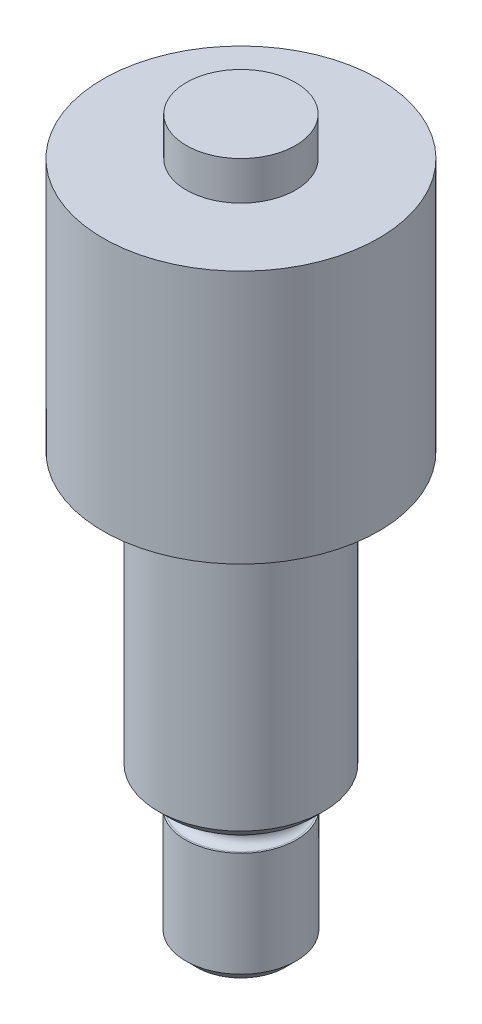
from build123d import *

# Parameters (mm, degrees)
CHAMFER_1_SIZE = 2
FILLET_1_R     = 1
FILLET_2_R     = 1.5


with BuildPart() as part:
    # 草图1 → 旋转1 (revolve)
    with BuildSketch(Plane.XY, mode=Mode.PRIVATE) as revolve_1_sk:
        Polygon((0, 0), (9.9, 0), (9.9, -7), (25, -7), (25, -53), (15, -53), (15, -104), (8.2, -104), (8.2, -109), (10, -109), (10, -130), (0, -130), align=None)
    revolve(revolve_1_sk.sketch.rotate(Axis((0, -130, 0), (0, 1, 0)), 90), axis=Axis((0, -130, 0), (0, 1, 0)))

    # 倒角1
    chamfer_1_edges = [part.edges().sort_by_distance(p)[0] for p in [
        (0, -104, 15),
        (0, -130, 10),
    ]]
    chamfer(chamfer_1_edges, length=CHAMFER_1_SIZE)

    # 圆角1
    fillet_1_edges = [part.edges().sort_by_distance(p)[0] for p in [
        (0, -53, 15),
    ]]
    fillet(fillet_1_edges, radius=FILLET_1_R)

    # 圆角2
    fillet_2_edges = [part.edges().sort_by_distance(p)[0] for p in [
        (0, -109, 8.2),
        (0, -104, 8.2),
    ]]
    fillet(fillet_2_edges, radius=FILLET_2_R)


solid = part.part
